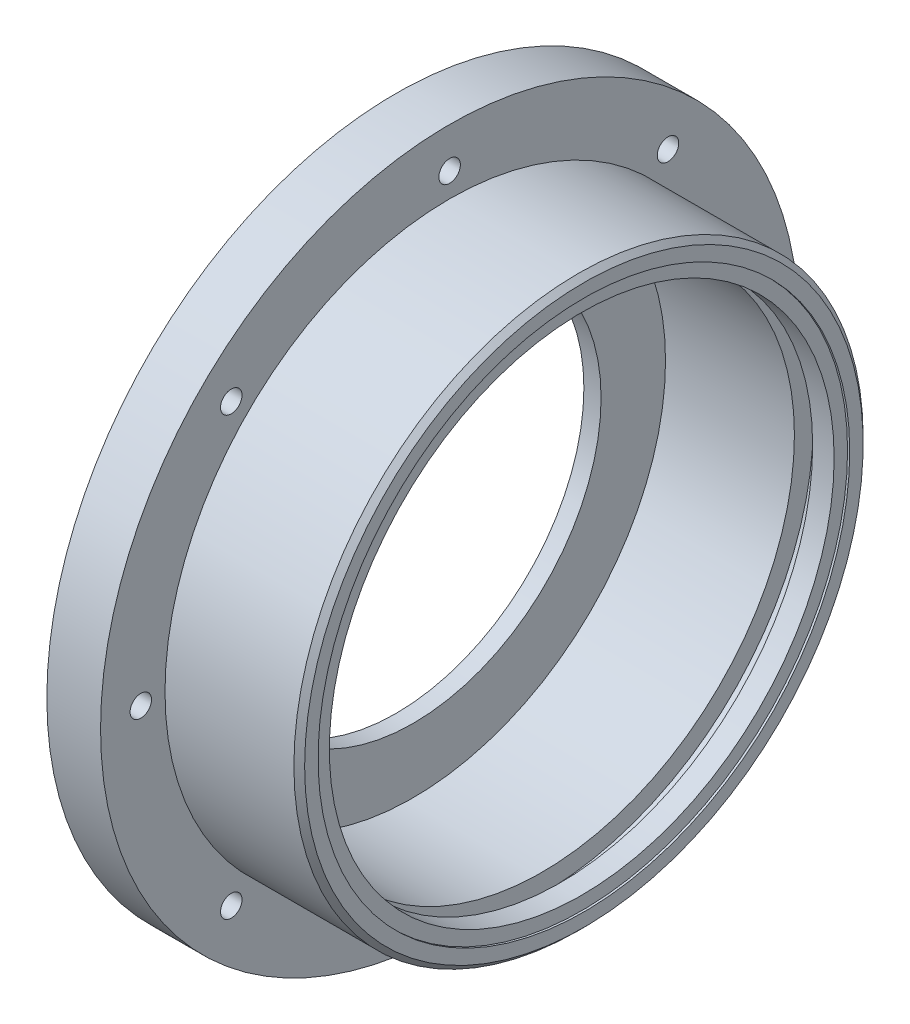
SolidWorks part; units mm, degrees
material "6061-T6 (SS)"
ref_plane "前视基准面" through (0, 0, 0) normal (0, 0, 1) x (1, 0, 0)
ref_plane "上视基准面" through (0, 0, 0) normal (0, 1, 0) x (1, 0, 0)
ref_plane "右视基准面" through (0, 0, 0) normal (1, 0, 0) x (0, 0, -1)
other "Configuration Table"
sketch "草图2" plane through (0, 0, 0) normal (0, 0, 1) x (1, 0, 0)
  line L0 (0, 0) -> (20, 0)
  dimension "D1" = 20
revolve "旋转-薄壁1" add sketch "草图2" angle 360 about L0 wall 65
sketch "草图3" plane through (0, 0, 0) normal (0, 0, 1) x (1, 0, 0)
  line L0 (20, 0) -> (45, 0)
  line L1 (20, -65) -> (20, 65) construction
  dimension "D1" = 25
revolve "旋转-薄壁2" add sketch "草图3" angle 360 about L0 wall 53
sketch "草图6" plane through (0, 0, 0) normal (1, 0, 0) x (0, 0, -1)
  circle A0 centre (0, 0) radius 35
  dimension "D1" = 70
extrude "切除-拉伸1" cut sketch "草图6" along normal through all
sketch "草图7" plane through (0, 0, 0) normal (1, 0, 0) x (0, 0, -1)
  circle A0 centre (0, 0) radius 47
  dimension "D1" = 94
extrude "切除-拉伸2" cut sketch "草图7" along normal through all from offset 13.2
sketch "草图10" plane through (0, 0, 0) normal (1, 0, 0) x (0, 0, -1)
  circle A0 centre (0, 0) radius 50.5
  dimension "D1" = 101
extrude "切除-拉伸4" cut sketch "草图10" against normal blind 3.4 from offset 40.6
sketch "草图12" plane through (0, 0, 0) normal (1, 0, 0) x (0, 0, -1)
  circle A0 centre (0, 0) radius 49.5
  dimension "D1" = 99
sketch "草图15" plane through (0, 0, 0) normal (1, 0, 0) x (0, 0, -1)
  circle A0 centre (0, 0) radius 65
extrude "切除-拉伸6" cut sketch "草图15" along normal blind 10
extrude "切除-拉伸5" cut sketch "草图12" along normal through all from offset 44.6
sketch "草图16" plane through (10, 0, 0) normal (-1, 0, 0) x (0, 0, 1)
  circle A2 centre (0, 57.5) radius 2
  circle A3 centre (40.6586, 40.6586) radius 2
  circle A4 centre (57.5, 0) radius 2
  circle A5 centre (40.6586, -40.6586) radius 2
  circle A6 centre (0, -57.5) radius 2
  circle A7 centre (-40.6586, -40.6586) radius 2
  circle A8 centre (-57.5, 0) radius 2
  circle A9 centre (-40.6586, 40.6586) radius 2
  point P20 (0, 0)
  dimension "D1" = 4
  dimension "D2" = 8
extrude "切除-拉伸7" cut sketch "草图16" against normal through all
chamfer "倒角1" distance 1 angle 45 1 edges at (45, 0, 53)
